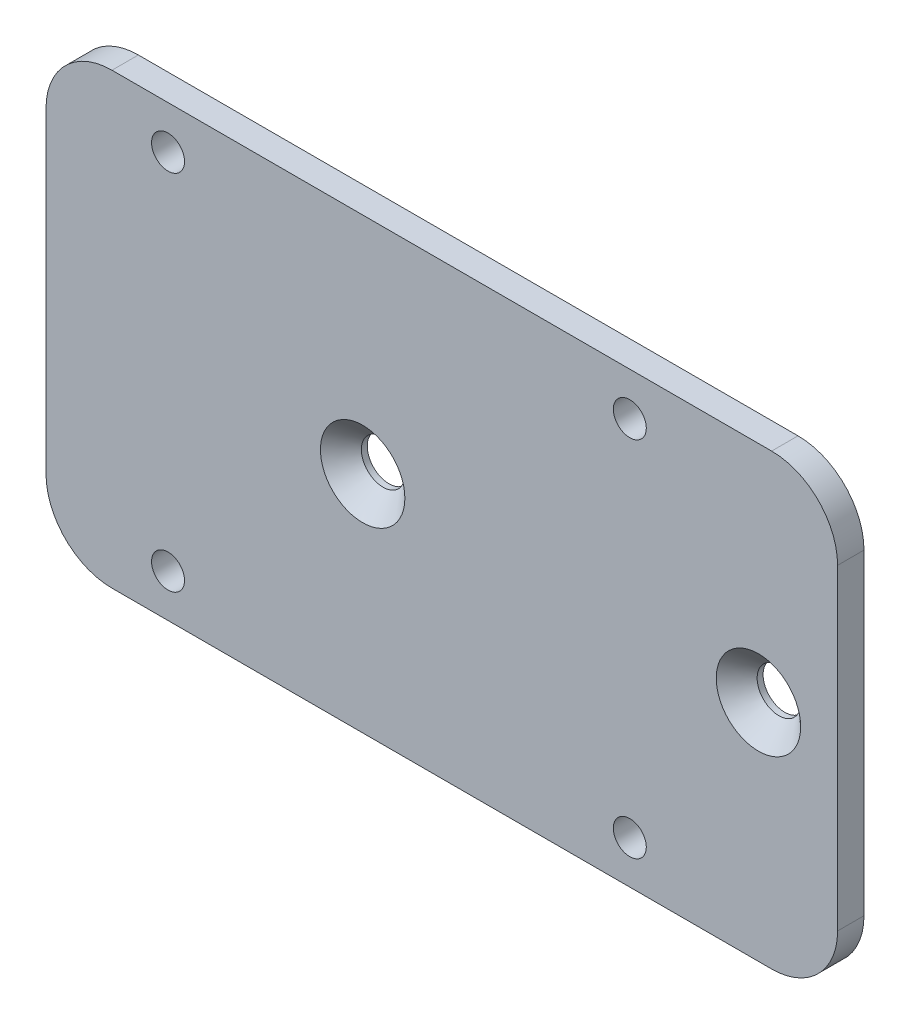
from build123d import *

# Parameters (mm, degrees)
SKETCH_1_W               = 120
SKETCH_1_H               = 68
EXTRUDE_1_DEPTH          = 4
HOLE_WIZARD_M6_1_D       = 5
FILLET_1_R               = 10
HOLE_WIZARD_3_AT_2_COUNT = 2
HOLE_WIZARD_3_AT_2_PITCH = 60


with BuildPart() as part:
    # 草图1 → 凸台-拉伸1 (new body)
    with BuildSketch(Plane.XY):
        Rectangle(SKETCH_1_W, SKETCH_1_H)
    extrude(amount=EXTRUDE_1_DEPTH)

    # M6 螺纹孔1 (through all)
    with Locations(Plane.XY.offset(4)):
        with Locations((28.49999693, -27.500007889), (-41.499997526, 27.499992111), (-41.499997526, -27.500007889), (28.49999693, 27.499992111)):
            Hole(HOLE_WIZARD_M6_1_D / 2)

    # 圆角1
    fillet_1_edges = [part.edges().sort_by_distance(p)[0] for p in [
        (60, -34, 2),
        (-60, -34, 2),
        (-60, 34, 2),
        (60, 34, 2),
    ]]
    fillet(fillet_1_edges, radius=FILLET_1_R)

    # 草图9 → 打孔尺寸(%根据)内六角花形半沉头螺钉的类型3 (revolve, cut)
    with BuildSketch(Plane(origin=(-12, 0, 4), x_dir=(0, -1, 0), z_dir=(1, 0, 0))):
        Polygon((0, 0), (0, 4), (3.3, 4), (3.3, 3.1), (6.4, 0), align=None)
    hole_wizard_3 = revolve(axis=Axis((-12, 0, 10.35), (0, 0, -1)), mode=Mode.SUBTRACT)

    # 打孔尺寸(%根据)内六角花形半沉头螺钉的类型3 at 2: 打孔尺寸(%根据)内六角花形半沉头螺钉的类型3 ×2
    with Locations(*[(i * HOLE_WIZARD_3_AT_2_PITCH, 0, 0) for i in range(1, HOLE_WIZARD_3_AT_2_COUNT)]):
        add(hole_wizard_3, mode=Mode.SUBTRACT)


solid = part.part
